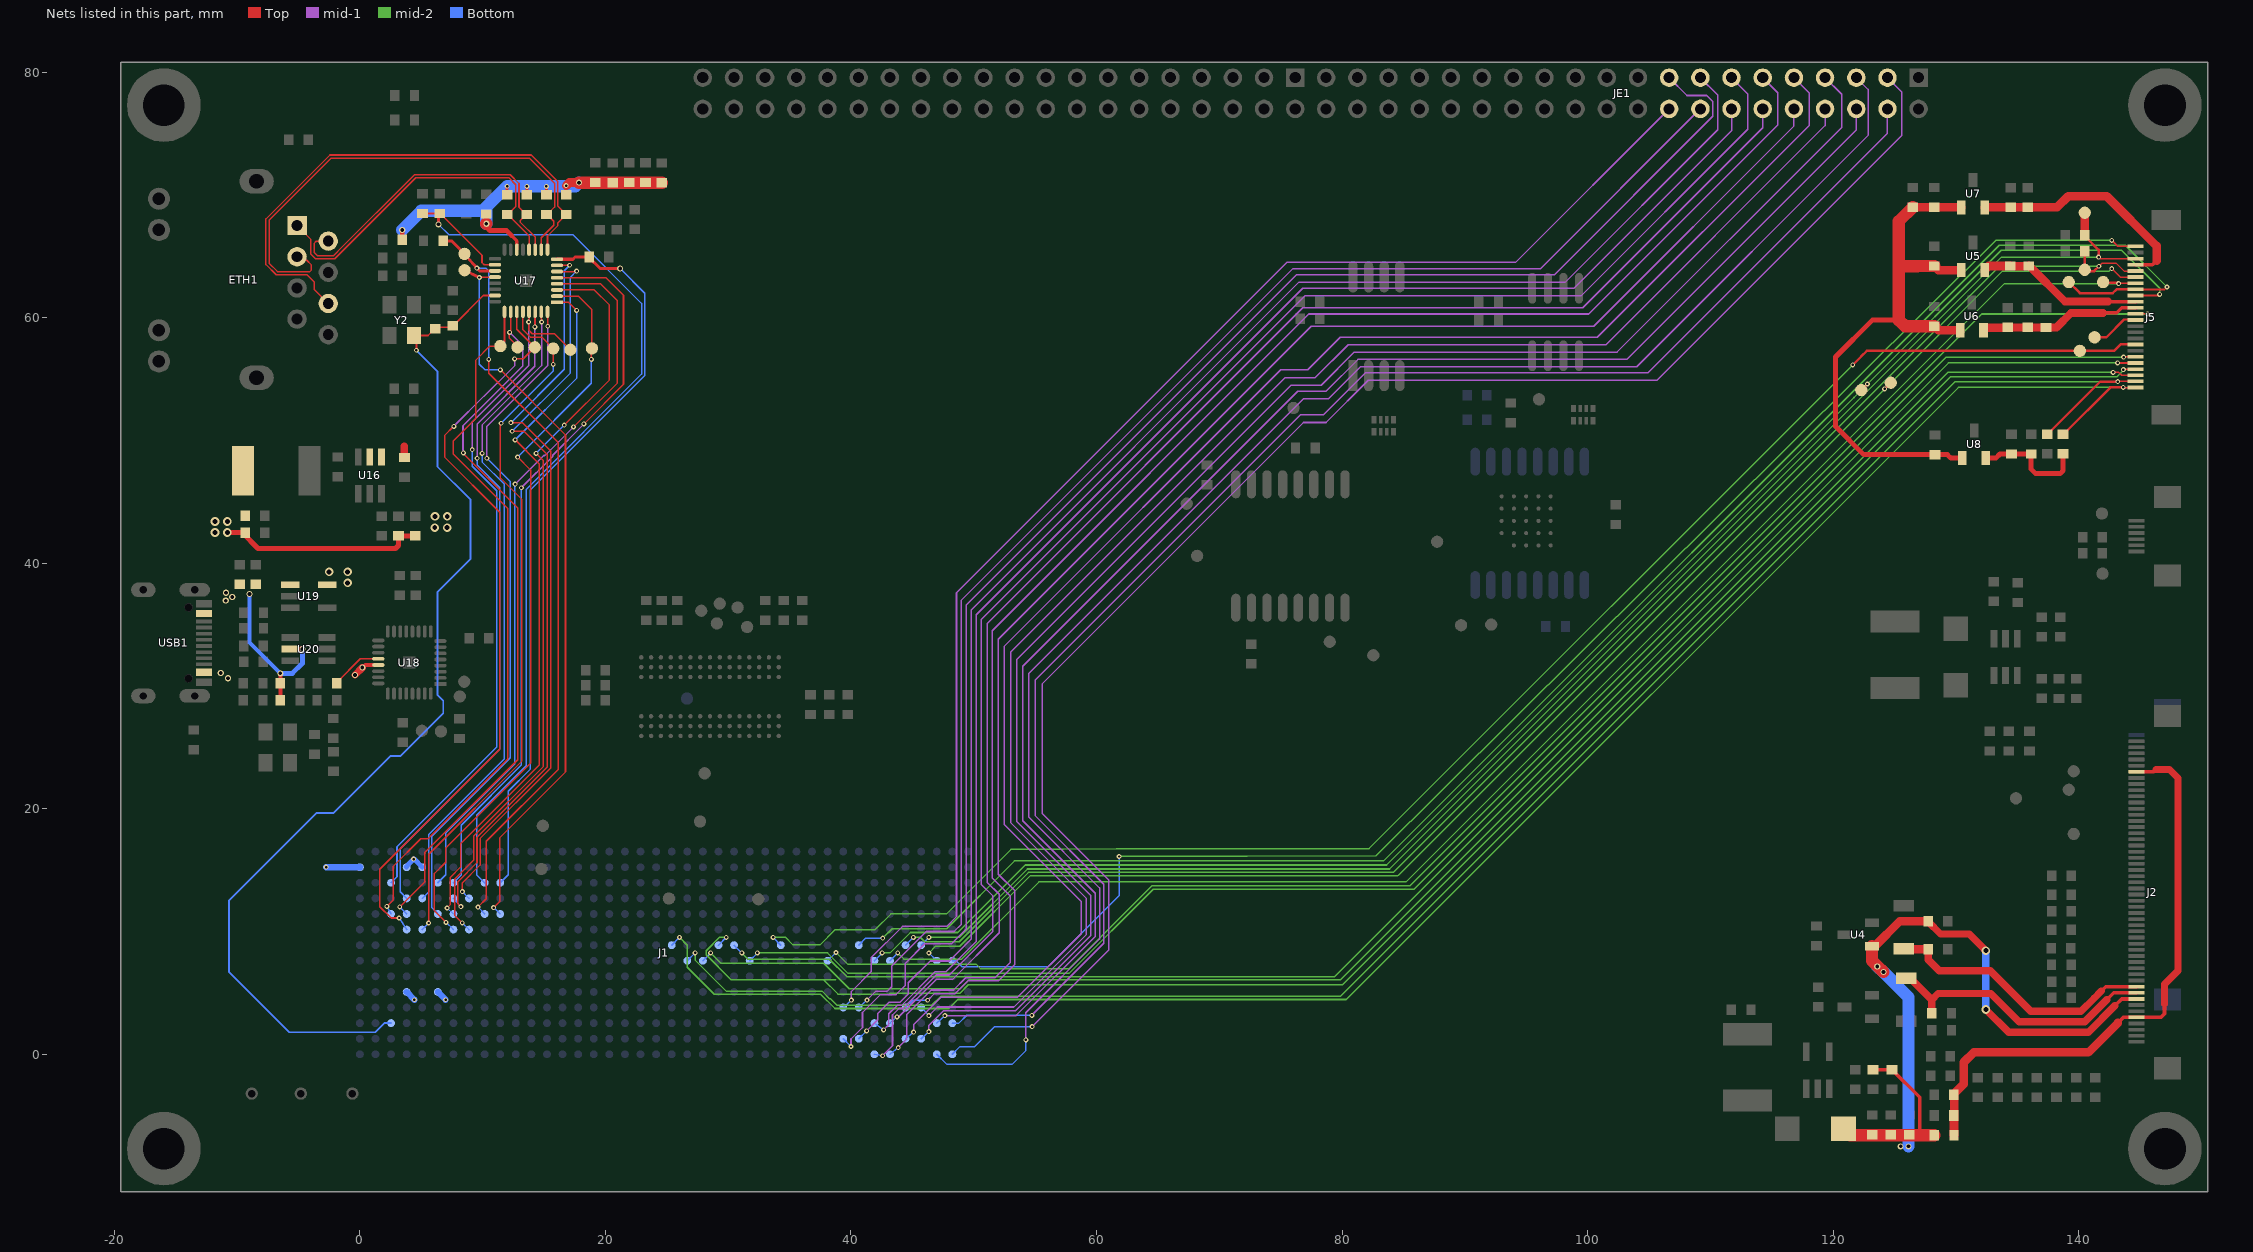
[diagram p0: the nets of this part, all layers, seen from the top]
# Altium PCB MISC105414.PcbDoc (part 4 of 11)
Units mm, origin at the board's own origin, x right, y up, seen from the top; angles counter-clockwise.
Board outline 170 x 92 mm, 6 copper layers (Top, GND, mid-1, mid-2, mid-3, Bottom), stack 1.231 mm thick; 238 components, 304 nets, 1456 pads, 1258 vias.
Unrouted connection lines stored in the file: 57.

## Via types
v1: diameter 0.4, hole 0.2, Top to Bottom, tented top, 618 vias
v2: diameter 0.5, hole 0.3, Top to Bottom, tented top, 522 vias
v3: diameter 0.5, hole 0.3, Top to Bottom, 41 vias
v4: diameter 1, hole 0.5, Top to Bottom, tented top, 36 vias
v5: diameter 0.7, hole 0.4, Top to Bottom, tented top, 34 vias
v6: diameter 1.3, hole 1.3, Top to Bottom, tented top, 3 vias
v7: diameter 4, hole 4, Top to Bottom, tented top, 2 vias
v8: diameter 3.3, hole 3.3, Top to Bottom, tented top, 2 vias

## Nets (pads, with @x,y where several pads share a name; then routed paths per layer and width w, separated by ;. In a path a pad name is that pad's centre, name@x,y a point inside that pad or via, vN(x,y) a via of type N, cw(c..) or ccw(c..) an arc to the next point about the centre after c; other vN are vias at no path point) (continued)
+3_3V_ETH: C71.1 C74.2 C78.2 C90.2 C91.2 LR5.1 LR7.1 R38.2 R43.2 R44.2 R45.2 U17.14 | length 41.2
  Top w0.25: v1(11.994,70.708) 11.994,70 R38.2@12,70 ; 12.361,66.682 12.78,66.263 U17.14@12.78,65.538 ; R43.2@13.6,70 v1(13.6,70.7) ; v1(15.191,70.689) 15.191,70 R44.2@15.2,70 ; R45.2@16.8,70 16.803,70 v1(16.803,70.752)
  Top w0.4: v2(3.45,67.15) 3.45,66.34 LR7.1@3.452,66.34 ; C91.2@10.286,68.452 10.286,67.65 10.286,67.4 10.595,67.091 11.952,67.091 12.361,66.682 ; C74.2@20.6,71.013 C74.2@20.6,71 C71.1@21.934,71 ; LR5.1@24.6,71 24.6,71.014 C78.2@23.267,71.014 ; C71.1@21.934,71 C71.1@21.934,71.014 ; C71.1@21.934,71 21.934,70.833 C71.1@21.934,71 ; C71.1@21.934,71 C71.1@21.934,71.014 ; C71.1@21.934,71.014 21.934,71.061 23.267,71.061 C78.2@23.267,71.014 ; C78.2@23.267,71 C78.2@23.267,71.014 ; C78.2@23.267,71 23.267,70.833 C78.2@23.267,71 ; C78.2@23.267,71 C78.2@23.267,71.014
  Top w0.7: v1(16.803,70.752) 17.063,71.013 C74.2@20.6,71.013
  Top w1: v2@10.286,67.65 v2(10.3,67.65) ; v2(17.85,71) C74.2@20.6,71 21.134,71 21.934,71 23.267,71 LR5.1@24.6,71
  Bottom w1: v2(3.45,67.15) 5,68.7 10.3,68.7 ; v2(10.3,67.65) 10.3,68.7 ; v1(13.6,70.7) v1@13.608,70.708 ; v1(15.191,70.689) v1@15.172,70.708 ; v2(17.85,71) 17.558,70.708 v1@15.172,70.708 ; 10.3,68.7 10.3,69.013 v1(11.994,70.708) v1@13.608,70.708 ; v1@13.608,70.708 v1@15.172,70.708
+3_3VO: C88.1 U18.20 | length 4.2
  Top w0.127: C88.1@-1.892,30.236 -1.892,30.287 0.032,32.21 U18.20@1.502,32.21
+4V_VCOM: C22.1 J2.6 J2.46 R21.1 R22.2 | length 47.7
  Top w0.3: 143.2,2.55 143.66,3.01 J2.46@144.73,3.01 146.71,3.01 147,3.3 147,4.1 ; J2.6@144.73,23.01 146.11,23.01 146.3,23.2
  Top w0.6: 146.3,23.2 147.4,23.2 148.1,22.5 148.1,6.8 147,5.7 147,4.1
  Top w0.7: R22.2@129.838,-4.988 R22.2@129.85,-4.988 ; R21.1@129.85,-6.6 R22.2@129.85,-4.988 ; 143.2,2.55 140.8,0.15 131.45,0.15 130.65,-0.65 130.65,-2.425 129.838,-3.237 C22.1@129.838,-3.288 129.869,-3.288 129.869,-3.37 129.869,-4.906 129.869,-4.988 R22.2@129.85,-4.988
+5V: C81.1 C84.1 C87.2 L3.2 R30.1 U18.21 U19.5 | length 18.6
  Top w0.3: 0.464,31.71 U18.21@1.502,31.71
  Top w0.4: v5(-10.8,42.5) -9.597,42.5 -8.297,41.2 2.9,41.2 3.146,41.446 C81.1@3.146,42.225 R30.1@4.521,42.225
  Top w0.6: v2(-0.4,30.9) v2(0.2,31.5)
  other v5: -1,38.4 -2.5,39.3 -1,39.3 -11.8,42.5 -11.8,43.4 -10.8,43.4
+5V_USB: C92.1 C93.1 R35.2 R36.2 U19.1 U20.5 USB1.2 USB1.11 | length 14
  Top w0.3: v2(-6.475,31.025) v2(-6.475,31.025) R35.2@-6.474,30.236 R36.2@-6.474,28.836
  Top w0.4: U20.5@-5.67,33.01 v2(-4.67,33.01)
  Bottom w0.3: v2(-8.992,37.5) -8.992,33.542 v2(-6.475,31.025)
  Bottom w0.4: v2(-6.475,31.025) -5.5,31.025 -4.689,31.836 -4.689,32.991 v2(-4.67,33.01)
  other v2: -10.75,30.625 -11.339,31.054 -10.925,36.95 -10.4,37.25 -10.9,37.6
+10_4V_AVDD: C14.2 C16.2 C17.1 C18.1 C19.2 D2.2 J2.43 R19.2 R21.2 U4.1 | length 64.5
  Top w0.3: R19.2@123.25,-1.25 123.301,-1.25 124.749,-1.25 C14.2@124.8,-1.25 127.05,-3.5 127.05,-6.35 126.85,-6.55 C19.2@126.2,-6.55 ; 142.95,3.95 143.51,4.51 J2.43@144.73,4.51
  Top w0.6: C16.2@127.75,10.85 127.75,10.799 128.749,9.8 131.1,9.8 v5(132.45,8.45) ; v5(132.45,3.65) 134.3,1.8 140.8,1.8 142.95,3.95
  Top w0.7: U4.1@123.175,8.8 123.4,8.8 125.45,10.85 C16.2@127.75,10.85
  Top w1: D2.2@120.85,-6.05 121.4,-6.6 R21.2@128.25,-6.6 ; U4.1@123.175,8.8 123.175,7.625 123.625,7.175 v2(124.1,6.7)
  Bottom w0.6: v5(132.45,3.65) v5(132.45,8.45)
  Bottom w1: v2(123.6,7.15) v2(124.1,6.7) 126.15,4.65 v2(126.15,-7.5)
  other v2: 125.5,-7.5
+12V: C69.1 J1.C35 J1.C37 J1.L36 J1.L37 J1.L40 U16.4 U16.5 | length 7.4
  Top w0.6: 3.625,49.55 3.625,48.627 C69.1@3.637,48.616
  Bottom w0.4: J1.L37@3.81,15.24 3.81,15.305 3.93,15.425 3.93,15.457 v1(4.378,15.905) 4.415,15.905 J1.L36@5.08,15.24
  Bottom w0.5: v1(-2.75,15.25) -2.74,15.24 J1.L40@0,15.24 ; J1.C37@3.81,5.08 v1(4.445,4.445) ; J1.C35@6.35,5.08 v1(6.985,4.445)
  other v5: 6.1,42.9 7.1,42.9 6.116,43.816 7.116,43.816
+16V_VGH: C21.1 DZ1.1 J2.41 | length 22.5
  Top w0.3: 141.85,5.15 142.21,5.51 J2.41@144.73,5.51
  Top w0.6: C21.1@127.75,8.55 127.75,7.7 128.65,6.8 132.8,6.8 136.1,3.5 140.2,3.5 141.25,4.55 141.85,5.15
  Top w0.7: DZ1.1@125.75,8.6 125.75,8.55 C21.1@127.75,8.55
-7V_VGL: C20.1 DZ2.2 J2.42 | length 22.7
  Top w0.3: 142.3,4.45 142.86,5.01 J2.42@144.73,5.01
  Top w0.6: DZ2.2@125.95,6.2 126.3,6.2 128.05,4.45 ; C20.1@128.05,3.35 128.05,4.45 ; 142.3,4.45 140.5,2.65 135.15,2.65 132.85,4.95 128.55,4.95 128.05,4.45
DVP_AFVDD: C34.1 C38.2 R24.1 U8.2 | length 9.3
  Top w0.4: U8.2@132.434,48.561 133.261,48.561 133.594,48.894 C34.1@134.53,48.894 134.581,48.894 136.079,48.894 C38.2@136.13,48.894 136.13,47.67 136.5,47.3 138.496,47.3 138.73,47.534 R24.1@138.73,48.91
DVP_AVDD: C33.1 C37.2 J5.4 U7.2 | length 20.5
  Top w0.3: J5.4@144.63,64.31 146.01,64.31 146.35,64.65
  Top w0.7: U7.2@132.35,68.975 132.35,68.99 C33.1@134.47,68.99 ; C37.2@135.87,68.99 C33.1@134.47,68.99 ; 146.35,64.65 146.35,65.85 142.3,69.9 139.16,69.9 138.25,68.99 C33.1@134.47,68.99
DVP_D0: J1.F20 J5.24 R24.2 | length 150.4
  Top w0.127: v1(143.634,54.323) 143.634,54.31 J5.24@144.63,54.31
  Top w0.2: R24.2@138.73,50.51 138.781,50.51 142.594,54.323 v1(143.634,54.323)
  mid-2 w0.127: v1(26.035,9.525) 26.673,8.887 26.673,7.08 28.856,4.897 37.527,4.897 38.694,3.73 47.959,3.73 48.69,4.462 80.35,4.462 130.211,54.323 v1(143.634,54.323)
  Bottom w0.127: J1.F20@25.4,8.89 v1(26.035,9.525)
DVP_D1: J1.E19 J5.23 R23.2 | length 148.9
  Top w0.127: v1(143.189,54.79) 143.189,54.81 J5.23@144.63,54.81
  Top w0.2: R23.2@137.43,50.51 137.481,50.51 141.761,54.79 v1(143.189,54.79)
  mid-2 w0.127: v1(27.305,8.255) 27.305,7.675 29.828,5.151 37.632,5.151 38.261,4.523 38.329,4.523 38.867,3.984 46.584,3.984 47.316,4.716 79.851,4.716 129.924,54.79 v1(143.189,54.79)
  Bottom w0.127: J1.E19@26.67,7.62 v1(27.305,8.255)
DVP_D2: J1.E15 J5.19 | length 134.6
  Top w0.127: v1(143.665,56.789) 143.665,56.81 J5.19@144.63,56.81
  mid-2 w0.127: v1(32.385,8.255) 38.092,8.255 39.761,6.586 57.767,6.586 64.623,13.442 85.87,13.442 129.218,56.789 v1(143.665,56.789)
  Bottom w0.127: J1.E15@31.75,7.62 v1(32.385,8.255)
DVP_D3: J1.F17 J5.21 | length 143.2
  Top w0.127: v1(143.647,55.776) 143.647,55.81 J5.21@144.63,55.81
  mid-2 w0.127: v1(29.845,9.525) 29.3,9.525 28.212,8.436 28.212,8.104 30.237,6.079 37.768,6.079 ; 38.768,6.079 37.768,6.079 ; v1(143.647,55.776) 143.647,55.725 143.1,55.178 129.551,55.178 80.034,5.66 49.563,5.66 48.873,4.97 43.182,4.97 43.119,4.908 38.939,4.908 37.768,6.079
  Bottom w0.127: J1.F17@29.21,8.89 v1(29.845,9.525)
DVP_D4: J1.E18 J5.22 | length 139.1
  Top w0.127: v1(142.817,55.544) 143.272,55.544 143.507,55.31 J5.22@144.63,55.31
  mid-2 w0.127: v1(28.575,8.255) 29.407,7.423 37.783,7.423 39.87,5.336 48.88,5.336 49.608,6.065 79.868,6.065 129.347,55.544 v1(142.817,55.544)
  Bottom w0.127: J1.E18@27.94,7.62 v1(28.575,8.255)
DVP_D5: J1.F16 J5.20 | length 135.9
  Top w0.127: v1(143.176,56.318) 143.176,56.31 J5.20@144.63,56.31
  mid-2 w0.127: v1(31.115,8.255) 31.619,7.751 38.237,7.751 39.655,6.332 79.411,6.332 129.397,56.318 v1(143.176,56.318)
  Bottom w0.127: J1.F16@30.48,8.89 v1(31.115,8.255)
DVP_D9: J1.E10 J5.12 | length 131.4
  Top w0.127: J5.12@144.63,60.31 145.6,60.31 v1(145.6,60.3)
  mid-2 w0.127: v1(38.783,8.292) 39.726,7.349 50.182,7.349 50.546,6.985 57.785,6.985 64.541,13.741 85.545,13.741 85.582,13.779 132.104,60.3 v1(145.6,60.3)
  Bottom w0.127: J1.E10@38.1,7.62 v1(38.783,8.292)
DVP_DOVDD: C32.1 C36.2 J5.11 R25.1 U6.2 | length 13.3
  Top w0.3: 142,60.4 143.1,60.4 143.51,60.81 J5.11@144.63,60.81
  Top w0.65: C32.1@134.243,59.217 135.846,59.217 C36.2@135.846,59.208 137.343,59.208 R25.1@137.343,59.203 138.2,59.203 139.397,60.4 142,60.4
  Top w0.7: U6.2@132.25,58.975 132.25,59.188 134.243,59.188 C32.1@134.243,59.217
DVP_DVDD: C31.1 C35.2 J5.10 U5.2 | length 13.7
  Top w0.3: 142.4,61.3 143.01,61.31 J5.10@144.63,61.31
  Top w0.65: C35.2@135.946,64.208 135.997,64.208 138.905,61.3 142.4,61.3
  Top w0.7: U5.2@132.35,63.875 132.683,64.208 C31.1@134.446,64.208 134.446,64.177 134.528,64.177 135.864,64.177 135.946,64.177 C35.2@135.946,64.208
DVP_HSYNC: J1.E7 J5.9 TP12.1 | length 134.7
  Top w0.127: J5.9@144.63,61.81 146.51,61.81 v1(146.6,61.9)
  Top w0.2: TP12.1@122.3,54.1 v1(122.8,54.6)
  mid-2 w0.127: v1(42.545,8.255) 43.18,8.255 44.846,9.921 48.693,9.921 54.192,15.42 83.629,15.42 121.704,53.496 ; v1@122.804,54.596 121.704,53.496 ; v1(146.6,61.9) 146.6,62.404 143.504,65.5 133.7,65.5 v1(122.8,54.6) 121.704,53.504 121.704,53.496
  Bottom w0.127: J1.E7@41.91,7.62 v1(42.545,8.255)
DVP_MCLK: J5.13 TP16.1 | length 4
  Top w0.2: TP16.1@141.3,58.4 142.249,58.4 143.7,59.851 144.63,59.851 J5.13@144.63,59.81
DVP_PCLK: J1.F13 J5.17 TP17.1 | length 132.4
  Top w0.2: v1(121.6,56.15) 122.312,56.862 122.312,56.871 122.741,57.3 TP17.1@140.1,57.3 142.89,57.3 143.441,57.851 144.63,57.851 J5.17@144.63,57.81
  mid-2 w0.127: v1(33.655,9.525) 34.668,9.525 35.283,8.91 37.485,8.91 38.711,10.136 41.966,10.136 43.26,11.43 47.777,11.43 53.028,16.681 61.593,16.729 62.105,16.729 82.205,16.755 v1(121.6,56.15)
  Bottom w0.127: v1(33.655,9.525) J1.F13@34.29,8.89
DVP_PWDN: J1.F8 J5.8 TP11.1 | length 140.2
  Top w0.127: J5.8@144.63,62.31 144.63,62.294 146.994,62.294 v1(147.2,62.5)
  Top w0.2: TP11.1@139.2,62.9 140.1,62 142.78,62 143.09,62.31 J5.8@144.63,62.31
  mid-2 w0.127: v1(42.594,9.464) 43.354,10.225 47.801,10.225 53.287,15.711 53.324,15.748 83.386,15.748 133.538,65.9 143.8,65.9 v1(147.2,62.5)
  Bottom w0.127: J1.F8@40.64,8.89 41.214,9.464 v1(42.594,9.464)
DVP_RST: J1.E3 J5.6 TP15.1 | length 123.3
  Top w0.127: v1(142.7,64) 143.39,63.31 J5.6@144.63,63.31
  Top w0.2: v1(124.2,54.2) TP15.1@124.7,54.7
  mid-2 w0.127: v1(46.35,8.25) 46.897,8.797 48.865,8.797 54.624,14.556 84.556,14.556 84.593,14.593 v1(124.2,54.2) 133.8,63.8 142.5,63.8 v1(142.7,64)
  Bottom w0.127: v1(46.35,8.25) J1.E3@46.99,7.62
DVP_SCL: J1.F5 J5.5 R26.1 TP14.1 | length 126.6
  Top w0.127: v1(141.657,64.189) 141.917,64.45 143.05,64.45 143.706,63.794 144.63,63.794 J5.5@144.63,63.81
  Top w0.2: R26.1@140.5,65.4 TP14.1@140.5,63.9 140.6,63.8 141.267,63.8 v1(141.657,64.189)
  mid-2 w0.127: v1(45.085,9.525) 45.645,9.525 46.009,9.161 48.812,9.161 54.462,14.811 84.17,14.811 133.548,64.189 v1(141.657,64.189)
  Bottom w0.127: J1.F5@44.45,8.89 v1(45.085,9.525)
DVP_SDA: J1.F4 J5.3 R27.1 TP13.1 | length 126.3
  Top w0.127: v1(141.626,64.94) 141.757,64.81 J5.3@144.63,64.81
  Top w0.2: R27.1@140.5,66.7 140.5,66.649 141.626,65.523 v1(141.626,64.94)
  Top w0.7: R27.1@140.5,66.7 TP13.1@140.5,68.55
  mid-2 w0.127: v1(46.355,9.525) 48.813,9.525 54.379,15.091 83.87,15.091 133.72,64.94 v1(141.626,64.94)
  Bottom w0.127: J1.F4@45.72,8.89 v1(46.355,9.525)
DVP_STROBE: J1.E2 J5.1 | length 123
  Top w0.127: v1(142.7,66.3) 143.19,65.81 J5.1@144.63,65.81
  mid-2 w0.127: v1(61.849,16.111) 82.763,16.164 133.274,66.3 v1(142.7,66.3)
  Bottom w0.127: J1.E2@48.26,7.62 48.553,7.62 49.037,7.136 56.056,7.136 61.849,12.93 v1(61.849,16.111)
DVP_VCC: C27.1 C28.1 C29.1 C30.1 LR3.1 U5.1 U6.1 U7.1 U8.1 | length 47.7
  Top w0.4: 125.35,59.8 123.2,59.8 120.2,56.8 120.2,51.15 122.5,48.85 C30.1@128.3,48.85 129.314,48.85 129.602,48.561 U8.1@130.534,48.561
  Top w0.7: LR3.1@126.5,69 126.5,69.008 C29.1@128.246,69.008 130.45,69.008 U7.1@130.45,68.975 ; C28.1@128.246,59.308 128.579,58.975 U6.1@130.35,58.975 ; C27.1@128.246,64.208 128.579,63.875 U5.1@130.45,63.875
  Top w1: LR3.1@126.5,69 125.35,67.85 125.35,64.2 ; C28.1@128.246,59.308 125.85,59.308 125.35,59.8 125.35,64.2 ; C27.1@128.246,64.208 126.853,64.208 126.845,64.2 125.35,64.2
DVP_VSYNC: J1.E6 J5.7 TP10.1 | length 126.1
  Top w0.127: v1(143.253,62.777) 143.253,62.81 J5.7@144.63,62.81
  Top w0.2: TP10.1@142,62.9 142,62.839 143.253,62.839 v1@143.253,62.81
  mid-2 w0.127: v1(43.815,8.255) 44.315,7.755 49.024,7.755 55.311,14.041 85.22,14.041 133.956,62.777 v1(143.253,62.777)
  Bottom w0.127: J1.E6@43.18,7.62 v1(43.815,8.255)
ETH_CLK: C85.1 J1.A38 R33.2 U17.23 Y2.1 | length 87.1
  Top w0.15: Y2.1@4.4,58.55 Y2.1@4.6,58.55 ; v1(4.6,57.35) Y2.1@4.6,58.55 ; U17.23@11.002,61.81 10.06,61.81 7.601,59.35 C85.1@7.55,59.35 7.55,59.225 6.15,59.225 R33.2@6.15,59.1 6.099,59.1 5.549,58.55 Y2.1@4.6,58.55
  Bottom w0.15: J1.A38@2.54,2.54 1.99,2.54 1.25,1.8 -5.748,1.8 -10.668,6.72 -10.668,12.513 -3.513,19.668 -2.134,19.668 2.482,24.285 3.288,24.285 6.787,27.784 6.787,28.806 6.32,29.273 6.32,37.645 9,40.325 9,45.2 6.32,47.88 6.32,55.63 v1(4.6,57.35)
ETH_COL: J1.K38 TP44.1 U17.29 | length 57.5
  Top w0.127: U17.29@13.78,60.482 13.78,60.132 v1(13.75,59.65) 13.75,59 14.05,58.7 15.85,58.7 17.154,57.396 TP44.1@17.145,57.386
  mid-1 w0.127: v1(9.15,49.25) 9.15,51.5 13.75,56.1 v1(13.75,59.65)
  Bottom w0.127: J1.K38@2.54,13.97 3.024,14.454 3.024,16.9 11.146,25.022 11.146,45.9 9.15,47.896 v1(9.15,49.25)
ETH_CRS: J1.G37 TP45.1 U17.27 | length 61.5
  Top w0.127: v1(3.2,11.1) 2.55,11.1 1.625,12.025 1.625,15.075 11.4,24.85 11.4,44.15 6.9,48.65 6.9,50.4 v1(7.65,51.15) ; v1(12.6,56.65) 13.309,56.65 TP45.1@14.245,57.586 12.78,59.052 U17.27@12.78,60.482
  mid-1 w0.127: v1(7.65,51.15) 10.113,53.613 10.137,53.613 12.6,56.075 v1(12.6,56.65)
  Bottom w0.127: v1(3.2,11.1) J1.G37@3.81,10.16
ETH_INTN: J1.K31 R40.2 U17.8 | length 61.4
  Top w0.25: U17.8@16.058,64.76 17.337,64.76 17.52,64.943 R40.2@18.679,64.943 18.679,64.893 19.572,64 v2(21.2,64)
  Bottom w0.127: J1.K31@11.43,13.97 12.086,14.626 12.086,21.436 13.889,23.239 13.889,45.989 23.2,55.3 23.2,62 v2(21.2,64)
ETH_MDC: J1.H31 TP51.1 U17.20 | length 60.8
  Top w0.127: v1(9.733,63.273) 9.77,63.31 U17.20@11.002,63.31 ; v1(10.897,11.955) 11.375,12.433 11.375,17.625 16.75,23 16.75,50.45 v1(11.45,55.75)
  Top w0.25: TP51.1@8.533,63.866 v1(9.733,63.273)
  Bottom w0.127: v1(9.733,63.273) 9.733,56.2 10.183,55.75 v1(11.45,55.75) ; v1(10.897,11.955) J1.H31@11.43,11.43
ETH_MDIO: J1.H32 R42.2 TP50.1 U17.19 | length 64
  Top w0.127: v1(9.621,11.995) 10.3,12.675 10.3,17.354 16.15,23.204 16.15,49.825 10.5,55.475 v1(10.5,56.6)
  Top w0.25: R42.2@6.777,66.262 7.457,66.262 TP50.1@8.521,65.198 v1(9.534,64.039) 9.763,63.81 U17.19@11.002,63.81
  Bottom w0.127: v1(9.534,64.039) 10.25,64.039 10.5,63.789 v1(10.5,56.6) ; v1(9.621,11.995) J1.H32@10.16,11.43
ETH_RD_N: ETH1.6 R45.1 U17.9 | length 43.8
  Top w0.127: ETH1.6@-2.575,61.155 -3.706,62.286 -3.706,62.892 -4.313,63.499 -6.822,63.499 -7.654,64.331 -7.654,68.043 -2.443,73.254 13.959,73.254 16.112,71.101 16.112,69.088 R45.1@16.8,68.4 16.1,67.7 16.1,67.475 15.28,66.655 U17.9@15.28,65.538
ETH_RD_P: ETH1.3 R44.1 U17.10 | length 41.7
  Top w0.127: ETH1.3@-5.115,64.965 -4.838,64.688 -4.338,64.688 -3.95,64.3 -3.95,63.875 -4.07,63.755 -6.719,63.755 -7.4,64.436 -7.4,67.929 -2.329,73 13.8,73 15.857,70.943 15.857,69.006 R44.1@15.251,68.4 ; U17.10@14.78,65.538 14.78,66.515 15.8,67.534 15.8,67.851 R44.1@15.251,68.4 ; R44.1@15.2,68.4 R44.1@15.251,68.4
ETH_RESETN: C89.2 J1.K32 R41.2 U17.18 | length 81.1
  Top w0.127: R41.2@5.103,68.489 5.154,68.489 6.4,68.489 6.554,68.489 9.948,65.095 9.948,64.488 10.125,64.31 U17.18@11.002,64.31
  Top w0.25: v2(6.4,67.6) C89.2@6.4,68.489
  Bottom w0.127: v2(6.4,67.6) 7.25,66.75 17.35,66.75 22.946,61.154 22.946,55.405 13.55,46.009 13.55,23.5 9.529,19.479 9.529,14.601 J1.K32@10.16,13.97
ETH_RX_CLK: J1.H38 TP43.1 U17.25 | length 57.6
  Top w0.127: v1(2.2,12.05) 2.7,12.55 2.7,15.3 4.95,17.55 5.55,17.55 12.05,24.05 12.05,44.45 7.6,48.9 7.6,49.95 9.45,51.8 9.45,56.55 10.586,57.686 TP43.1@11.445,57.686 11.78,58.021 U17.25@11.78,60.482
  Bottom w0.127: v1(2.2,12.05) J1.H38@2.54,11.43
ETH_RX_D0: J1.J37 U17.30 | length 54.1
  Top w0.127: v1(14.25,59.25) 14.265,59.25 14.265,60.482 U17.30@14.28,60.482
  mid-1 w0.127: v1(9.55,48.55) 9.55,51.35 14.25,56.05 v1(14.25,59.25)
  Bottom w0.127: J1.J37@3.81,12.7 3.278,13.232 3.278,16.75 11.4,24.872 11.4,46.15 9.55,48 v1(9.55,48.55)
ETH_RX_D1: J1.J36 U17.31 | length 53.3
  Top w0.127: U17.31@14.78,60.482 14.78,60.132 v1(14.8,59.65)
  mid-1 w0.127: v1(9.95,48.95) 9.95,51.25 14.8,56.1 v1(14.8,59.65)
  Bottom w0.127: J1.J36@5.08,12.7 5.6,13.22 5.6,17.9 11.75,24.05 11.75,46.45 9.95,48.25 v1(9.95,48.95)
ETH_RX_D2: J1.H35 U17.32 | length 54.7
  Top w0.127: U17.32@15.28,60.482 15.3,60.462 v1(15.3,59.3)
  mid-1 w0.127: v1(10.35,48.55) 10.35,51.15 15.3,56.1 v1(15.3,59.3)
  Bottom w0.127: J1.H35@6.35,11.43 6.35,11.458 5.866,11.942 5.866,17.766 12.25,24.15 12.25,46.65 v1(10.35,48.55)
ETH_RX_D3: J1.H34 U17.1 | length 57.2
  Top w0.127: v1(7.1,11.917) 7.376,12.194 7.376,14.426 8.2,15.25 8.2,17.15 14.6,23.55 14.6,48.1 v1(12.65,50.05) ; U17.1@16.058,61.259 16.991,61.259 v1(17.65,60.6)
  Bottom w0.127: v1(7.1,11.917) J1.H34@7.62,11.43 ; v1(12.65,50.05) 17.65,55.05 v1(17.65,60.6)
ETH_RX_DV: J1.H37 TP41.1 U17.26 | length 59.1
  Top w0.127: v1(3.25,12) 5.3,14.05 5.3,16.45 12.85,24 12.85,44.5 8.432,48.918 v1(8.432,48.982) ; U17.26@12.28,60.482 12.28,58.88 v1(12.2,58.8) 12.16,58.76 12.16,58.353 12.523,57.99 TP41.1@12.886,57.627
  mid-1 w0.127: v1(8.432,48.982) 8.4,49.014 8.4,51.2 13.25,56.05 13.25,57.75 v1(12.2,58.8)
  Bottom w0.127: v1(3.25,12) J1.H37@3.81,11.43
ETH_RX_ER: J1.G36 TP42.1 U17.28 | length 57.8
  Top w0.127: v1(5.603,10.694) 5.603,16.303 13.2,23.9 13.2,45.182 11.45,46.932 11.45,51.35 v1(11.5,51.4) ; U17.28@13.28,60.482 13.28,59.02 13.9,58.4 14.832,58.4 TP42.1@15.745,57.486 15.748,57.486 15.748,56.2 v1(15.75,56.2)
  Bottom w0.127: J1.G36@5.08,10.16 v1(5.603,10.694) ; v1(11.5,51.4) 15.75,55.65 v1(15.75,56.2)
ETH_TD_N: ETH1.2 R43.1 U17.11 | length 28.2
  Top w0.127: ETH1.2@-2.575,66.235 -3.549,66.235 -3.734,66.05 -3.734,65.338 -3.45,65.054 -2.145,65.054 -1.825,65.375 -1.825,65.382 4.441,71.648 12.251,71.648 12.959,70.94 12.959,68.99 R43.1@13.549,68.4 ; R43.1@13.6,68.4 R43.1@13.549,68.4 ; U17.11@14.28,65.538 14.28,66.57 13.052,67.798 13.052,67.903 R43.1@13.549,68.4
ETH_TD_P: ETH1.1 R38.1 U17.12 | length 28.9
  Top w0.127: ETH1.1@-5.115,67.505 -3.988,66.378 -3.988,65.163 -3.625,64.8 -2.04,64.8 4.554,71.394 12.143,71.394 12.705,70.832 12.705,69.054 R38.1@12.051,68.4 ; R38.1@12,68.4 R38.1@12.051,68.4 ; U17.12@13.78,65.538 13.78,66.671 R38.1@12.051,68.4
ETH_TX_CLK: J1.G34 TP40.1 U17.2 | length 60.6
  Top w0.127: v1(7.015,10.751) 6.075,11.691 6.075,14.725 7,15.65 7,16.8 13.9,23.7 13.9,47.6 v1(12.85,48.65) ; U17.2@16.058,61.76 17.46,61.76 17.469,61.751 17.8,61.751 18.9,60.651 TP40.1@18.9,57.5 v1(18.85,56.6)
  Bottom w0.127: v1(7.015,10.751) J1.G34@7.62,10.16 ; v1(12.85,48.65) 18.85,54.65 v1(18.85,56.6)
ETH_TX_D0: J1.K35 U17.4 | length 59
  Top w0.127: U17.4@16.058,62.76 19.6,62.76 20.975,61.385 20.975,54.675 v1(17.4,51.1)
  mid-1 w0.127: v1(12.65,46.45) 14.975,48.775 15.075,48.775 v1(17.4,51.1)
  Bottom w0.127: J1.K35@6.35,13.97 7,14.62 7,18.016 12.6,23.616 12.6,46.4 v1(12.65,46.45)
ETH_TX_D1: J1.K34 U17.5 | length 59.6
  Top w0.127: U17.5@16.058,63.26 20.05,63.26 21.475,61.835 21.475,54.575 v1(18.25,51.35)
  mid-1 w0.127: v1(13.15,46.15) 15.7,48.7 15.7,48.8 v1(18.25,51.35)
  Bottom w0.127: J1.K34@7.62,13.97 8.255,14.605 8.255,18.664 13.15,23.559 v1(13.15,46.15)
ETH_TX_D2: J1.J34 U17.6 | length 61.4
  Top w0.127: v1(8.232,12.024) 7.988,12.268 7.988,14.063 9.538,15.613 9.538,17.679 15.25,23.391 15.25,48.875 13.375,50.75 v1(12.4,50.75) ; U17.6@16.058,63.76 17.65,63.76 v1(17.65,63.8)
  Bottom w0.127: J1.J34@7.62,12.7 v1(8.232,12.024) ; v1(12.4,50.75) 17.15,55.5 17.15,63.3 v1(17.65,63.8)
ETH_TX_D3: J1.J33 U17.7 | length 59.7
  Top w0.127: v1(8.352,13.247) 8.352,13.977 9.792,15.417 9.792,17.567 15.55,23.325 15.55,49.138 13.238,51.45 v1(12.3,51.45) ; U17.7@16.058,64.26 16.408,64.26 v1(17.091,64.27)
  Bottom w0.127: v1(8.352,13.247) J1.J33@8.89,12.7 ; v1(12.3,51.45) 16.65,55.8 16.65,63.829 v1(17.091,64.27)
ETH_TX_EN: J1.G33 U17.3 | length 61.8
  Top w0.127: v1(8.338,10.702) 7.734,11.306 7.734,14.284 9.284,15.834 9.284,17.784 9.3,17.8 14.95,23.45 14.95,48.35 v1(14.35,48.95) ; U17.3@16.058,62.26 19.1,62.26 20.325,61.035 20.325,54.925 v1(16.65,51.25)
  Bottom w0.127: v1(8.338,10.702) J1.G33@8.89,10.16 ; v1(14.35,48.95) v1(16.65,51.25)
EXT_IO0: J1.Y2 JE1.3 | length 133.9
  mid-1 w0.127: v1(54.75,2.25) 61,8.5 61,14.2 55.6,19.6 55.6,30.2 76.865,51.465 78.7,51.465 82.135,54.9 105.65,54.9 125.6,74.85 125.6,78.38 JE1.3@124.43,79.55
  Bottom w0.127: J1.Y2@48.26,0 48.885,0.625 50.075,0.625 51.7,2.25 v1(54.75,2.25)
EXT_IO1: J1.A2 JE1.4 | length 128.7
  mid-1 w0.127: v1(54.737,3.175) 60.6,9.038 60.6,13.85 55,19.45 55,30.476 76.624,52.1 78.5,52.1 81.9,55.5 104.9,55.5 124.43,75.03 JE1.4@124.43,77.01
  Bottom w0.127: J1.A2@48.26,2.54 48.795,2.54 49.43,3.175 v1(54.737,3.175)
EXT_IO2: J1.Y3 JE1.5 | length 135.2
  mid-1 w0.127: v1(54.25,1.175) 54.247,1.178 54.247,3.385 60.25,9.388 60.25,13.55 54.5,19.3 54.5,31.03 76.87,53.4 78.9,53.4 81.5,56 104,56 122.85,74.85 122.85,78.59 JE1.5@121.89,79.55
  Bottom w0.127: J1.Y3@46.99,0 47.79,-0.8 53.15,-0.8 54.25,0.3 v1(54.25,1.175)
EXT_IO3: J1.A3 JE1.6 | length 128
  mid-1 w0.127: v1(47.65,3.15) 53.45,3.15 59.9,9.6 59.9,13.125 54,19.025 54,31.6 76.4,54 78.7,54 81.3,56.6 103.2,56.6 121.89,75.29 JE1.6@121.89,77.01
  Bottom w0.127: J1.A3@46.99,2.54 v1(47.65,3.15)
EXT_IO4: J1.Z4 JE1.7 | length 132.3
  mid-1 w0.127: v1(46.35,1.85) 46.35,2.364 47.536,3.55 53.4,3.55 59.55,9.7 59.55,12.907 53.5,18.957 53.5,32.159 75.841,54.5 78.3,54.5 81,57.2 102.4,57.2 120.7,75.5 120.7,78.2 JE1.7@119.35,79.55
  Bottom w0.127: J1.Z4@45.72,1.27 v1(46.35,1.85)
EXT_IO5: J1.B4 JE1.8 | length 127.5
  mid-1 w0.127: v1(46.35,3.15) 47.05,3.85 53.275,3.85 59.15,9.725 59.15,12.725 53,18.875 53,32.75 75.35,55.1 77.8,55.1 80.5,57.8 101.5,57.8 119.35,75.65 JE1.8@119.35,77.01
  Bottom w0.127: J1.B4@45.72,3.81 v1(46.35,3.15)
EXT_IO6: J1.Z5 JE1.9 | length 131.7
  mid-1 w0.127: v1(45.1,1.8) 45.1,2.414 47.349,4.663 53.588,4.663 58.75,9.825 58.75,12.45 52.5,18.7 52.5,33.25 75,55.75 77.2,55.75 79.85,58.4 100.8,58.4 118.05,75.65 118.05,78.31 JE1.9@116.81,79.55
  Bottom w0.127: J1.Z5@44.45,1.27 v1(45.1,1.8)
EXT_IO7: J1.B5 JE1.10 | length 120.9
  mid-1 w0.127: v1(46.25,4.4) 46.768,4.918 48.461,4.918 49.519,5.975 51.995,5.975 53.34,7.32 53.34,13.335 52,14.675 52,33.8 77.5,59.3 100.5,59.3 116.81,75.61 JE1.10@116.81,77.01
  Bottom w0.127: J1.B5@44.45,3.81 45.04,4.4 v1(46.25,4.4)
EXT_IO8: J1.Y6 JE1.11 | length 127.1
  mid-1 w0.127: v1(43.85,0.55) 44.55,1.25 44.55,3.25 46.535,5.235 48.36,5.235 49.354,6.229 51.741,6.229 52.959,7.447 52.959,12.909 51.5,14.368 51.5,34.5 77.3,60.3 100.1,60.3 115.5,75.7 115.5,78.32 JE1.11@114.27,79.55
  Bottom w0.127: J1.Y6@43.18,0 v1(43.85,0.55)
EXT_IO9: J1.A6 JE1.12 | length 119
  mid-1 w0.127: v1(43.75,3.05) 43.9,3.05 46.948,6.098 48.262,6.098 52.07,9.906 52.07,13.03 51.1,14 51.1,35.1 76.8,60.8 99.6,60.8 114.27,75.47 JE1.12@114.27,77.01
  Bottom w0.127: J1.A6@43.18,2.54 v1(43.75,3.05)
EXT_IO10: J1.Y7 JE1.13 | length 124.9
  mid-1 w0.127: v1(42.572,-0.121) 43.386,0.694 43.386,3.201 43.914,3.728 44.213,3.728 46.943,6.458 48.006,6.458 51.562,10.014 51.562,12.888 50.6,13.85 50.6,35.4 77,61.8 99.5,61.8 113.05,75.35 113.05,78.23 JE1.13@111.73,79.55
  Bottom w0.127: J1.Y7@41.91,0 v1(42.572,-0.121)
EXT_IO11: J1.A7 JE1.14 | length 118.2
  mid-1 w0.127: v1(42.656,1.988) 43.084,2.416 43.084,3.295 43.771,3.982 44.108,3.982 46.843,6.717 47.738,6.717 50.2,9.179 50.2,35.8 76.8,62.4 98.9,62.4 111.73,75.23 JE1.14@111.73,77.01
  Bottom w0.127: J1.A7@41.91,2.54 v1(42.656,1.988)
EXT_IO12: J1.Z8 JE1.15 | length 122
  mid-1 w0.127: v1(41.275,1.905) 42.182,2.812 42.182,3.327 43.091,4.236 44.003,4.236 44.674,4.907 44.674,5.818 46.456,7.6 48,7.6 49.8,9.4 49.8,36.2 76.5,62.9 98.2,62.9 110.605,75.305 110.605,78.135 JE1.15@109.19,79.55
  Bottom w0.127: J1.Z8@40.64,1.27 v1(41.275,1.905)
EXT_IO13: J1.B8 JE1.16 | length 115.3
  mid-1 w0.127: v1(41.306,4.42) 42.01,5.123 42.945,5.123 43.326,5.504 43.326,7.2 46.126,10 48.4,10 49,10.6 49,37 76,64 96.18,64 JE1.16@109.19,77.01
  Bottom w0.127: J1.B8@40.64,3.81 v1(41.306,4.42)
EXT_IO14: J1.Z9 JE1.17 | length 125.6
  mid-1 w0.127: v1(40.005,0.635) 40.005,1.243 40.943,2.181 40.943,3.407 42.401,4.865 43.673,4.865 44.42,5.611 44.42,7.4 46.02,9 48.2,9 49.4,10.2 49.4,36.6 76.3,63.5 97.3,63.5 110.2,76.4 110.2,77.6 109.7,78.1 108.1,78.1 JE1.17@106.65,79.55
  Bottom w0.127: J1.Z9@39.37,1.27 v1(40.005,0.635)
EXT_IO15: J1.B9 JE1.18 | length 114.1
  mid-1 w0.127: v1(40.036,4.408) 40.036,5.116 41.656,6.736 41.656,7.88 44.194,10.418 47.8,10.418 48.6,11.218 48.6,37.6 75.5,64.5 94.14,64.5 JE1.18@106.65,77.01
  Bottom w0.127: J1.B9@39.37,3.81 v1(40.036,4.408)